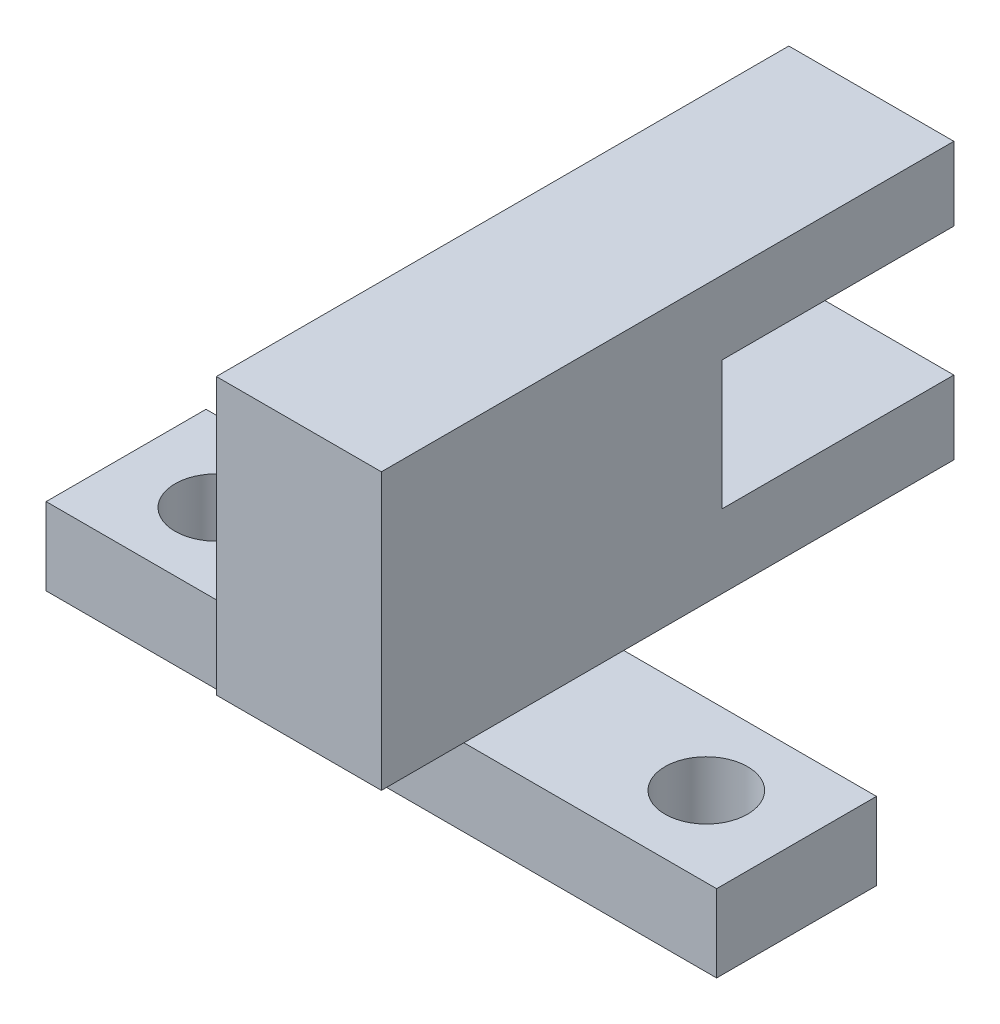
SolidWorks part; units mm, degrees
ref_plane "前视基准面" through (0, 0, 0) normal (0, 0, 1) x (1, 0, 0)
ref_plane "上视基准面" through (0, 0, 0) normal (0, 1, 0) x (1, 0, 0)
ref_plane "右视基准面" through (0, 0, 0) normal (1, 0, 0) x (0, 0, -1)
sketch "草图1" plane through (0, 0, 0) normal (0, 1, 0) x (1, 0, 0)
  line L1 (-13, 3.1) -> (13, 3.1)
  line L2 (-13, 3.1) -> (-13, -3.1)
  line L3 (-13, -3.1) -> (13, -3.1)
  line L4 (13, 3.1) -> (13, -3.1)
  line L5 (-13, 3.1) -> (13, -3.1) construction
  line L6 (-13, -3.1) -> (13, 3.1) construction
  point P0 (0, 0)
  dimension "D1" = 26
  dimension "D2" = 6.2
extrude "凸台-拉伸1" add sketch "草图1" along normal blind 3
sketch "草图2" plane through (0, 3, 0) normal (0, 1, 0) x (1, 0, 0)
  line L1 (-3.2, 15.9) -> (3.2, 15.9)
  line L2 (-3.2, 15.9) -> (-3.2, -6.3)
  line L3 (-3.2, -6.3) -> (3.2, -6.3)
  line L4 (3.2, 15.9) -> (3.2, -6.3)
  dimension "D1" = 3.2
  dimension "D2" = 3.2
  dimension "D3" = 6.3
  dimension "D4" = 22.2
extrude "凸台-拉伸2" add sketch "草图2" along normal blind 10.7
sketch "草图3" plane through (-3.2, 0, 0) normal (-1, 0, 0) x (0, 0, 1)
  line L0 (-15.9, 13.7) -> (-15.9, 3) construction
  line L1 (-15.9, 10.85) -> (-6.9, 10.85)
  line L2 (-15.9, 10.85) -> (-15.9, 5.85)
  line L3 (-15.9, 5.85) -> (-6.9, 5.85)
  line L4 (-6.9, 10.85) -> (-6.9, 5.85)
  line L5 (-15.9, 13.7) -> (6.3, 13.7) construction
  dimension "D1" = 9
  dimension "D2" = 5
  dimension "D3" = 2.85
extrude "切除-拉伸1" cut sketch "草图3" against normal blind 10.7
sketch "草图4" plane through (0, 3, 0) normal (0, 1, 0) x (1, 0, 0)
  circle A0 centre (-9.5, 0) radius 1.6
  circle A1 centre (9.5, 0) radius 1.6
  dimension "D1" = 3.2
  dimension "D2" = 3.2
  dimension "D3" = 9.5
  dimension "D4" = 9.5
extrude "切除-拉伸2" cut sketch "草图4" against normal blind 10.7
